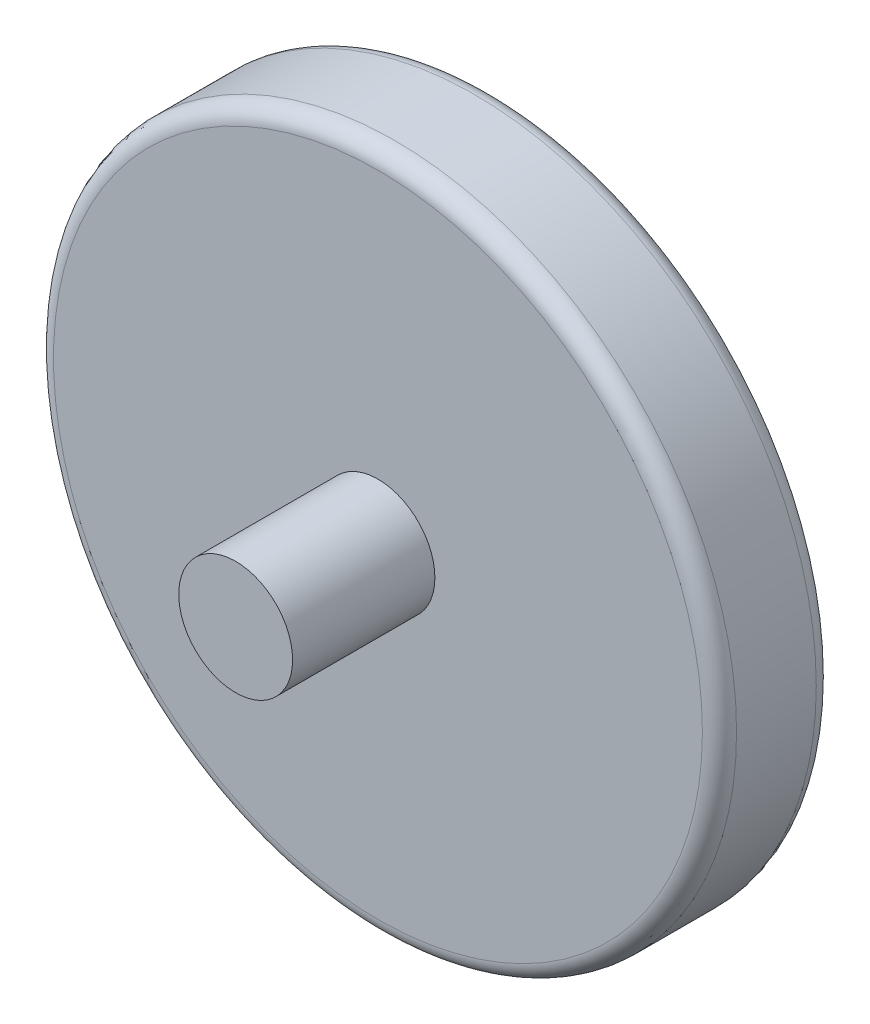
SolidWorks part; units mm, degrees
ref_plane "Front Plane" through (0, 0, 0) normal (0, 0, 1) x (1, 0, 0)
ref_plane "Top Plane" through (0, 0, 0) normal (0, 1, 0) x (1, 0, 0)
ref_plane "Right Plane" through (0, 0, 0) normal (1, 0, 0) x (0, 0, -1)
sketch "Sketch1" plane through (0, 0, 0) normal (0, 0, 1) x (1, 0, 0)
  circle A0 centre (0, 0) radius 60
  dimension "D1" = 120
extrude "Boss-Extrude1" add sketch "Sketch1" along normal blind 20
fillet "Fillet1" radius 3 2 edges at (60, 0, 0) (60, 0, 20)
sketch "Sketch2" plane through (0, 0, 0) normal (0, 0, -1) x (-1, 0, 0)
  circle A0 centre (0, 0) radius 10
  dimension "D1" = 20
extrude "Boss-Extrude2" add sketch "Sketch2" along normal blind 25
sketch "Sketch3" plane through (0, 0, 20) normal (0, 0, 1) x (1, 0, 0)
  circle A0 centre (0, 0) radius 10
  dimension "D1" = 20
extrude "Boss-Extrude3" add sketch "Sketch3" along normal blind 25
